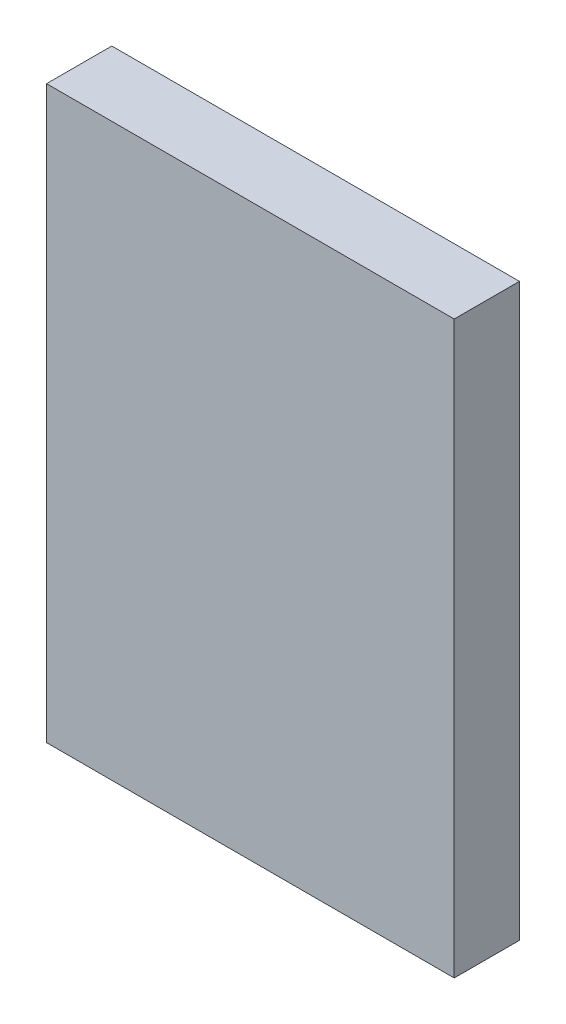
SolidWorks part; units mm, degrees
ref_plane "前视基准面" through (0, 0, 0) normal (0, 0, 1) x (1, 0, 0)
ref_plane "上视基准面" through (0, 0, 0) normal (0, 1, 0) x (1, 0, 0)
ref_plane "右视基准面" through (0, 0, 0) normal (1, 0, 0) x (0, 0, -1)
sketch "草图1" plane through (0, 0, 0) normal (0, 0, 1) x (1, 0, 0)
  line L1 (-25, -35) -> (25, -35)
  line L2 (-25, -35) -> (-25, 35)
  line L3 (-25, 35) -> (25, 35)
  line L4 (25, -35) -> (25, 35)
  line L5 (-25, -35) -> (25, 35) construction
  line L6 (-25, 35) -> (25, -35) construction
  point P0 (0, 0)
  dimension "D1" = 50
  dimension "D2" = 70
extrude "凸台-拉伸1" add sketch "草图1" along normal mid plane 8
